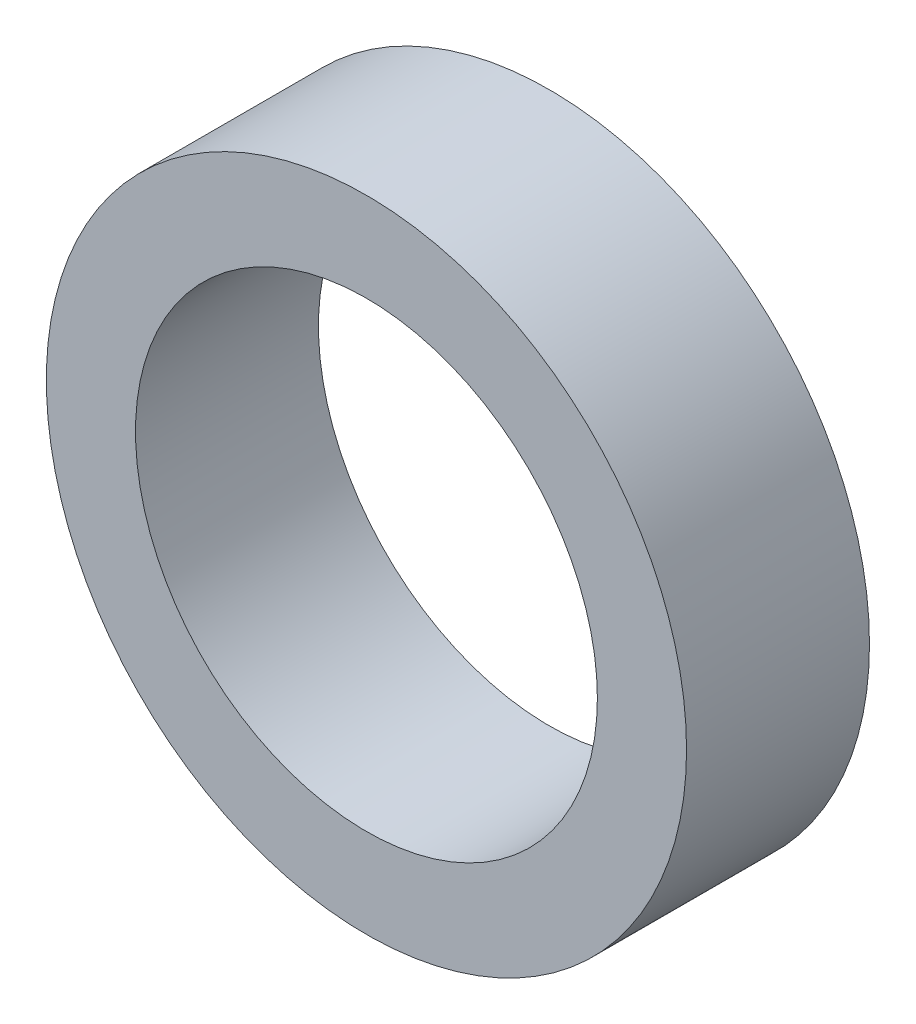
SolidWorks part; units mm, degrees
ref_plane "Front Plane" through (0, 0, 0) normal (0, 0, 1) x (1, 0, 0)
ref_plane "Top Plane" through (0, 0, 0) normal (0, 1, 0) x (1, 0, 0)
ref_plane "Right Plane" through (0, 0, 0) normal (1, 0, 0) x (0, 0, -1)
sketch "Sketch1" plane through (0, 0, 0) normal (0, 0, 1) x (1, 0, 0)
  circle A0 centre (0, 0) radius 10.1
  circle A1 centre (0, 0) radius 14
  dimension "D1" = 20.2
  dimension "D2" = 28
extrude "Boss-Extrude1" add sketch "Sketch1" along normal blind 8
